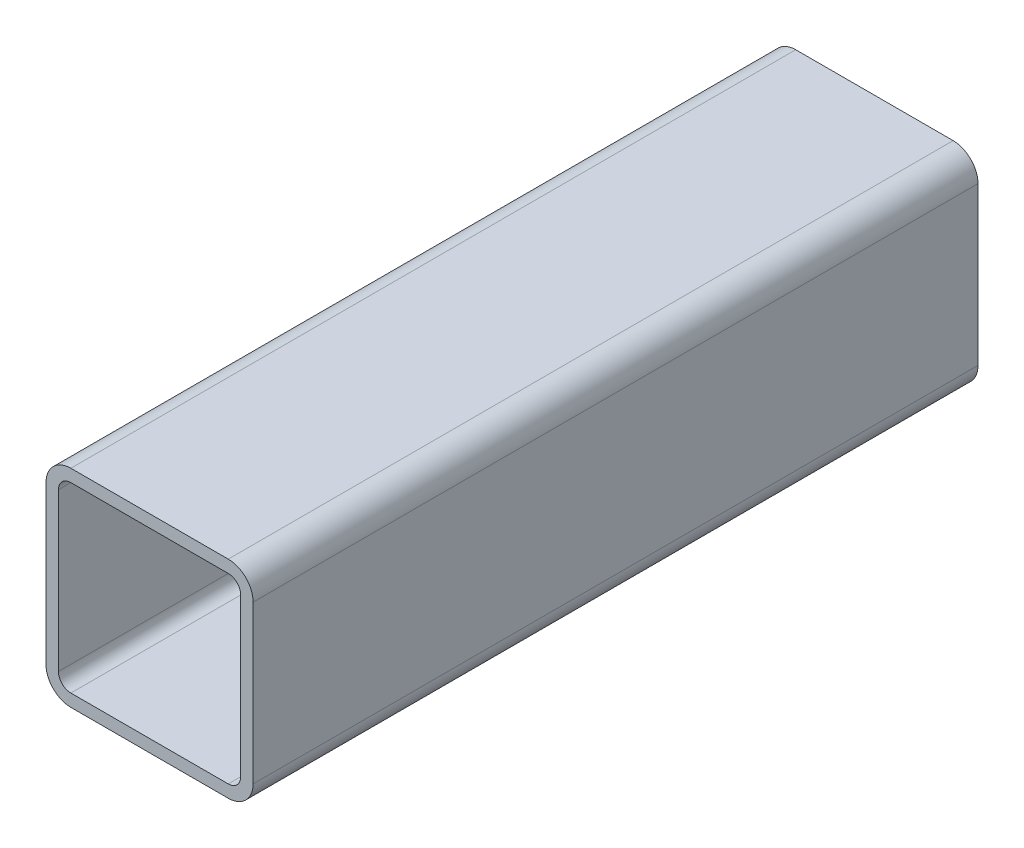
SolidWorks part; units mm, degrees
material "Q235B"
ref_plane "前视基准面" through (0, 0, 0) normal (0, 0, 1) x (1, 0, 0)
ref_plane "上视基准面" through (0, 0, 0) normal (0, 1, 0) x (1, 0, 0)
ref_plane "右视基准面" through (0, 0, 0) normal (1, 0, 0) x (0, 0, -1)
other "Configuration Table"
sketch "草图1" plane through (0, 0, 0) normal (1, 0, 0) x (0, 0, -1)
  line L0 (-87.5, 0) -> (87.5, 0)
other "Gb／6728-1986方形空心型钢 050 X 50 X 3(1)"
ref_plane "基准面1" through (0, 0, 87.5) normal (0, 0, -1) x (0, 1, 0)
sketch "Sketch1" plane through (0, 0, 87.5) normal (0, 0, -1) x (0, 1, 0)
  line L0 (-19, -22) -> (19, -22)
  line L1 (-22, -19) -> (-22, 19)
  line L2 (19, 22) -> (-19, 22)
  line L3 (22, 19) -> (22, -19)
  line L4 (-19, -25) -> (19, -25)
  line L5 (-25, -19) -> (-25, 19)
  line L6 (19, 25) -> (-19, 25)
  line L7 (25, 19) -> (25, -19)
  arc A0 (25, 19) -> (19, 25) centre (19, 19) ccw
  arc A1 (19, -25) -> (25, -19) centre (19, -19) ccw
  arc A2 (-25, -19) -> (-19, -25) centre (-19, -19) ccw
  arc A3 (-19, 25) -> (-25, 19) centre (-19, 19) ccw
  arc A4 (-19, 22) -> (-22, 19) centre (-19, 19) ccw
  arc A5 (22, 19) -> (19, 22) centre (19, 19) ccw
  arc A6 (19, -22) -> (22, -19) centre (19, -19) ccw
  arc A7 (-22, -19) -> (-19, -22) centre (-19, -19) ccw
  point P0 (-25, 0)
  point P1 (25, 0)
  point P2 (0, 25)
  point P3 (0, -25)
  point P4 (0, 0)
  point P5 (-25, -25)
  point P6 (25, -25)
  point P7 (25, 25)
  point P8 (-25, 25)
  point P33 (0, 0)
  dimension "D1" = 6
  dimension "Thickness" = 3
  dimension "V_leg" = 50
equation "\"D2@草图1\"=\"D1@草图1\"/2"
